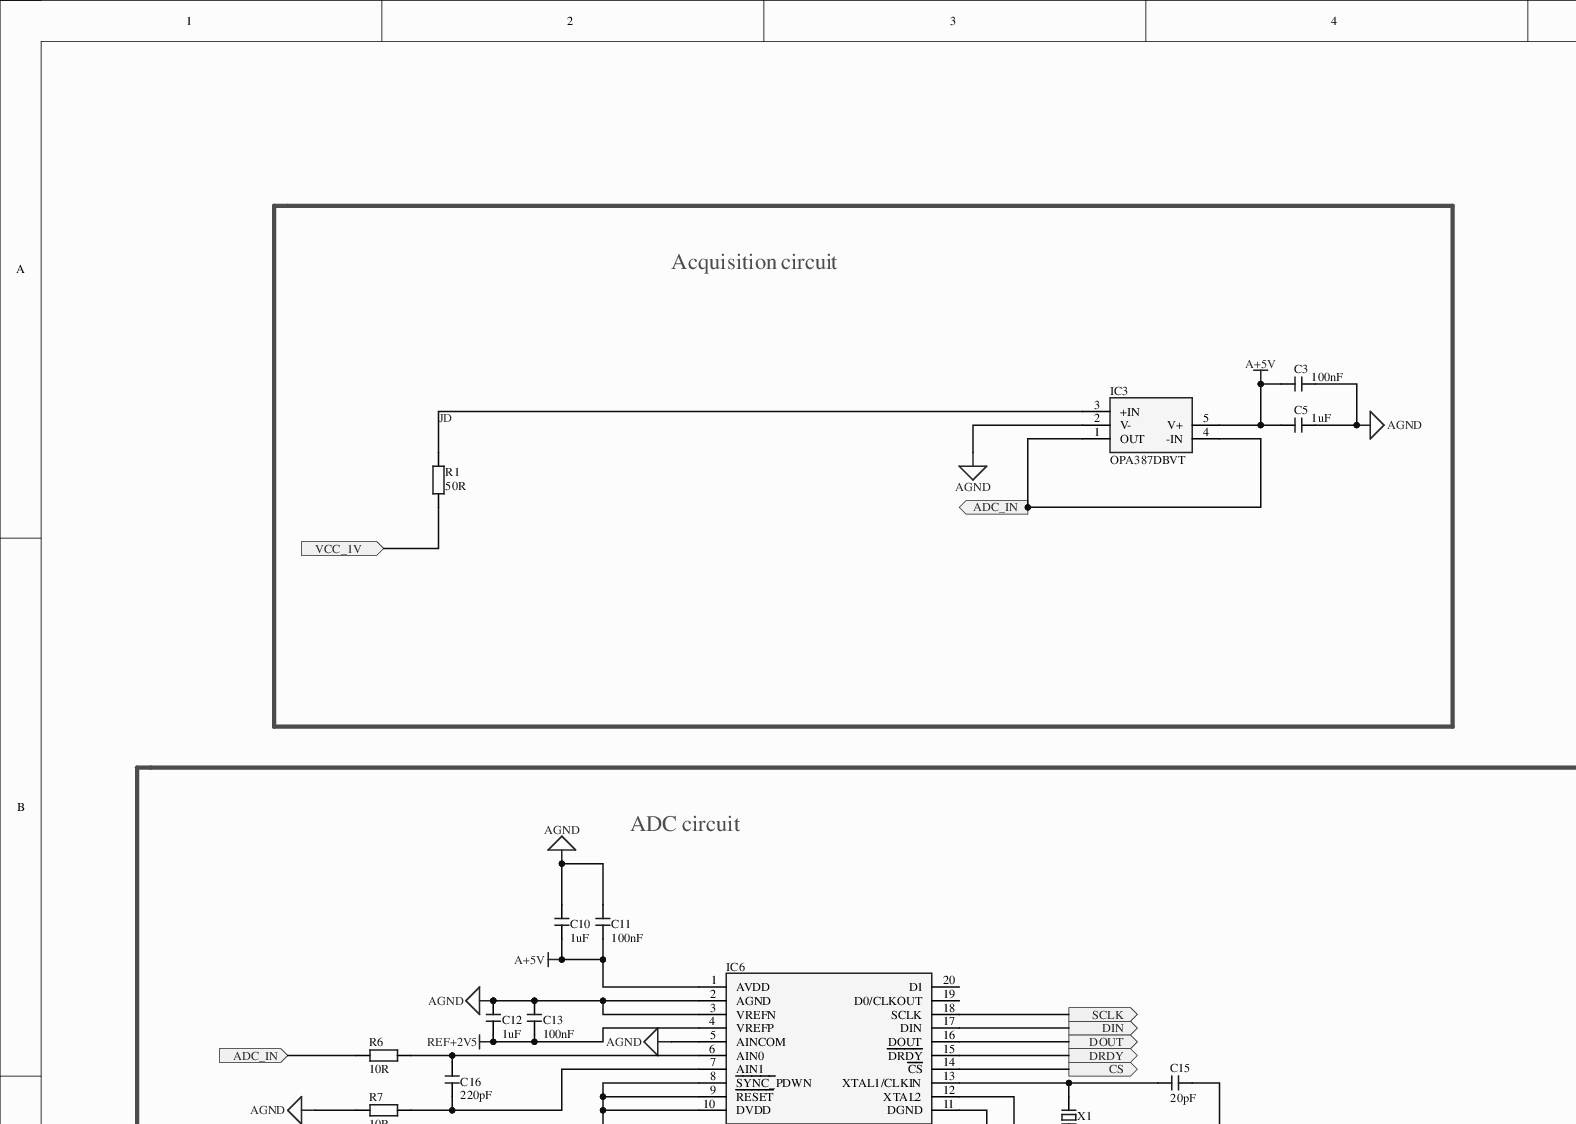
[diagram p0: MISC82306-4.SchDoc, top left]
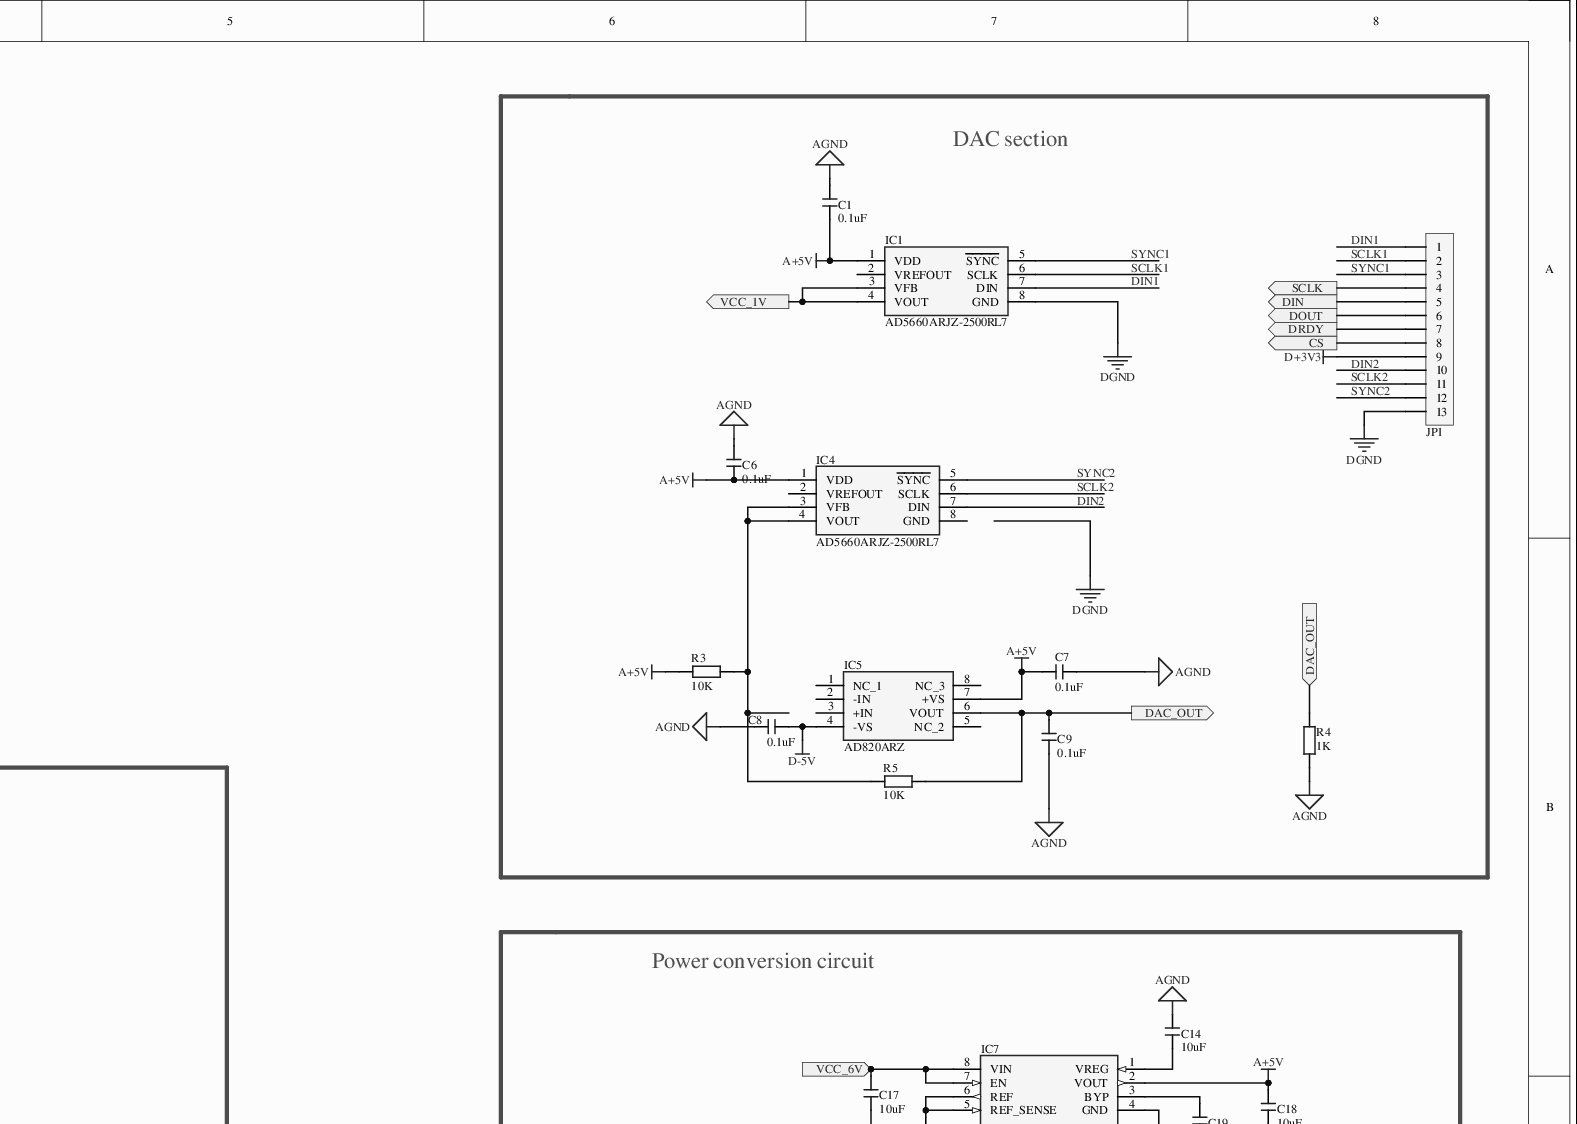
[diagram p1: MISC82306-4.SchDoc, top right]
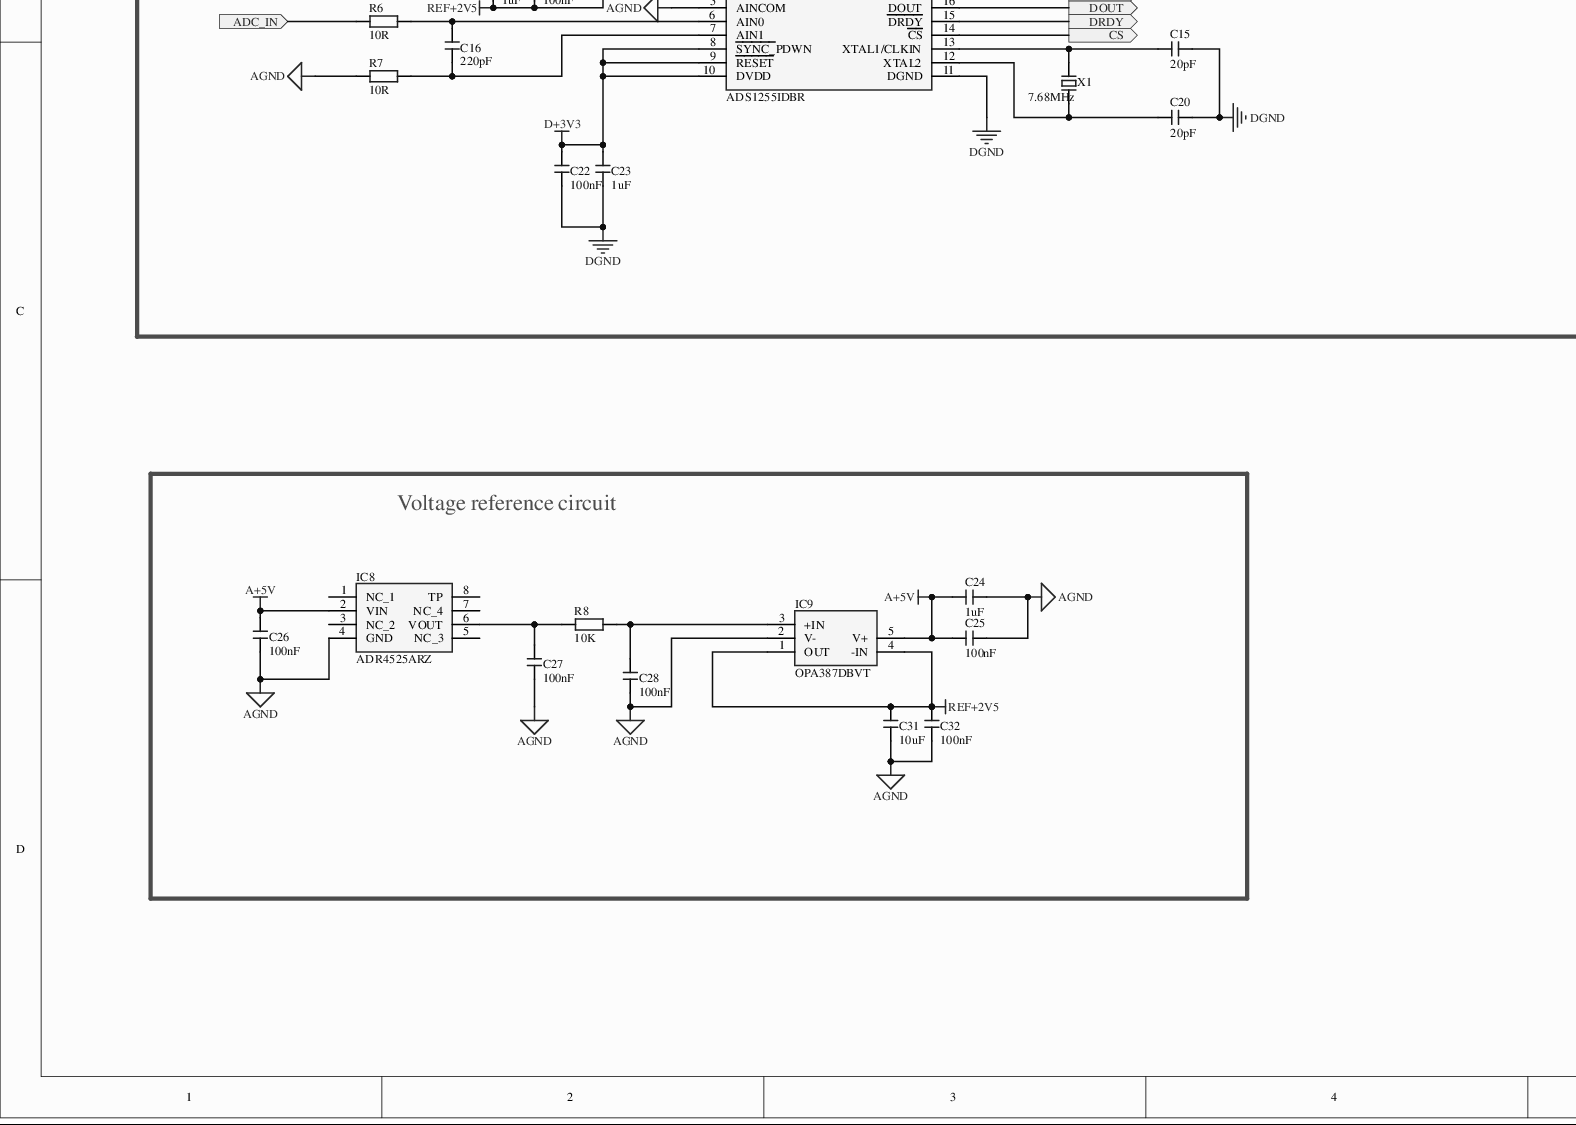
[diagram p2: MISC82306-4.SchDoc, bottom left]
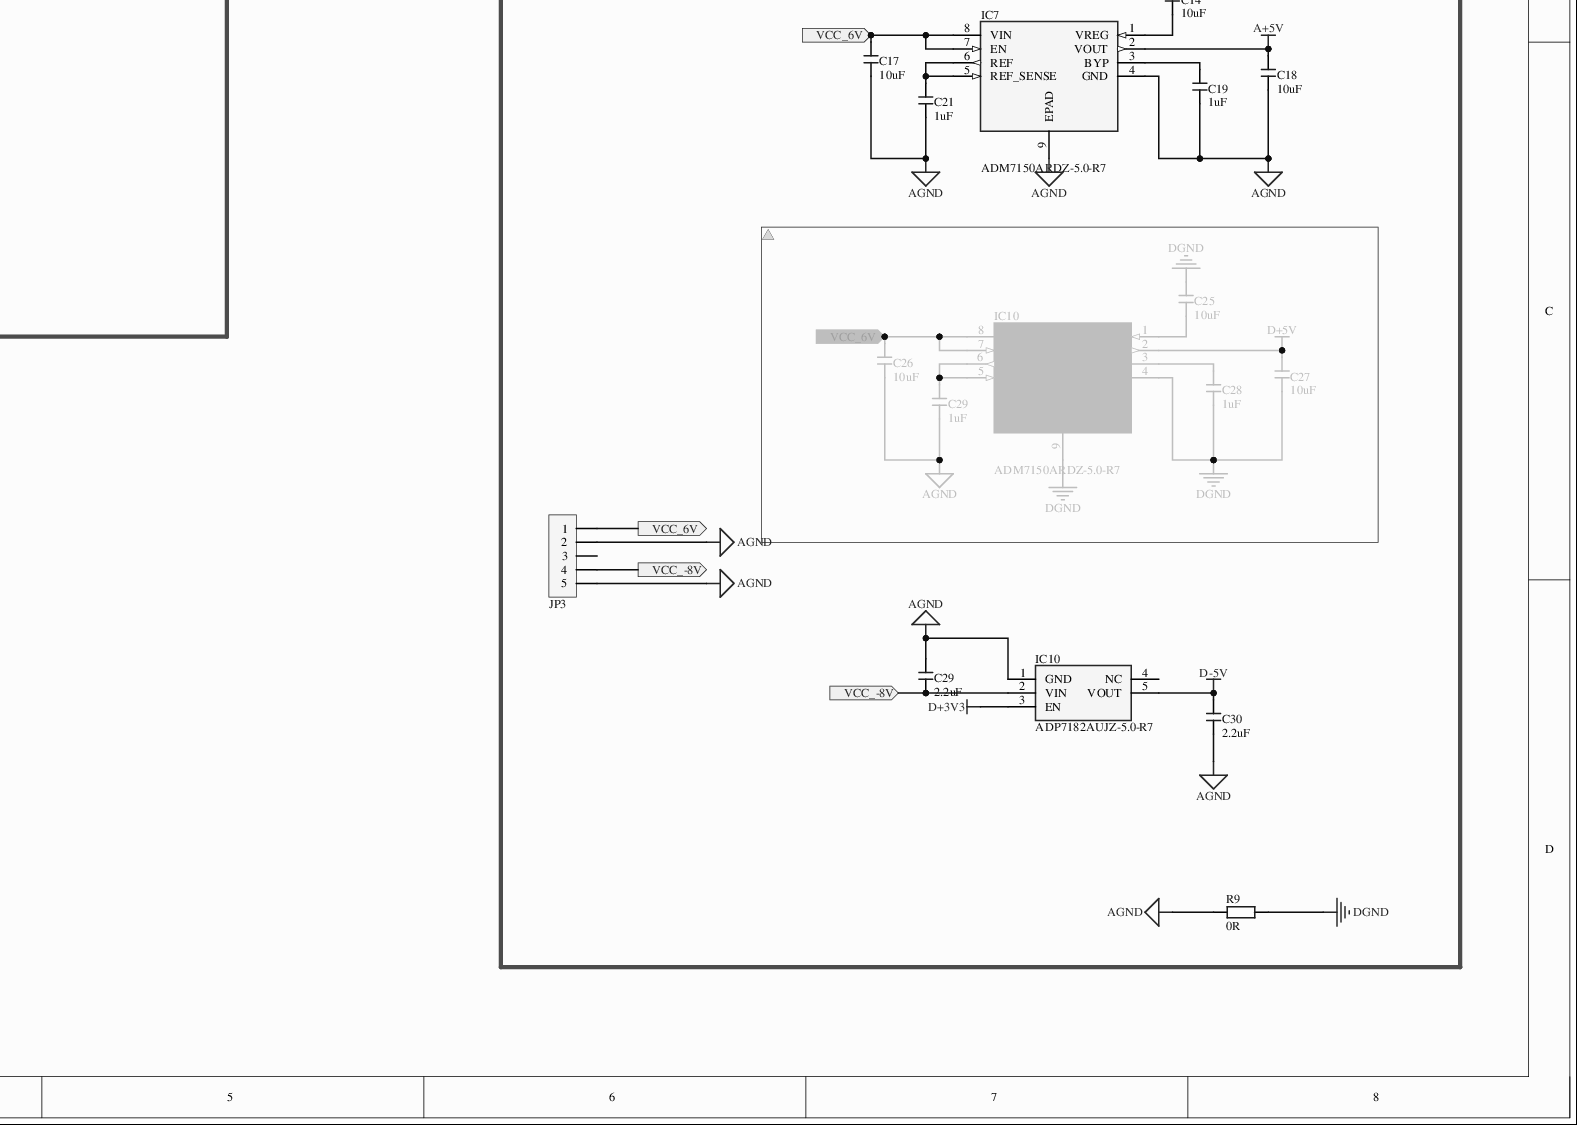
[diagram p3: MISC82306-4.SchDoc, bottom right]
# Altium project MISC82306-7.PrjPcb
1 sheet, 56 parts. Net scope: flat (ports and power ports of the same name join across sheets).
Board file: MISC82306.PcbDoc

## Sheet MISC82306-4.SchDoc
size A2

### Parts
(Parts that share a designator on the sheet are numbered #1, #2 ... from top to bottom, then left to right.)
C1  0.1uF  [C 0603_L]
C3  100nF  [C 0603_L]
C5  1uF  [C 0603_L]
C6  0.1uF  [C 0603_L]
C7  0.1uF  [C 0603_L]
C8  0.1uF  [C 0603_L]
C9  0.1uF  [C 0603_L]
C10  1uF  [C 0603_L]
C11  100nF  [C 0603_L]
C12  1uF  [C 0603_L]
C13  100nF  [C 0603_L]
C14  10uF  [C 0603_L]
C15  20pF  [C 0603_L]
C16  220pF  [C 0805_L]
C17  10uF  [C 0603_L]
C18  10uF  [C 0603_L]
C19  1uF  [C 0603_L]
C20  20pF  [C 0603_L]
C21  1uF  [C 0603_L]
C22  100nF  [C 0603_L]
C23  1uF  [C 0603_L]
C24  1uF  [C 0603_L]
C25#1  10uF  [C 0603_L]  (masked out: inside a compile mask, not in the netlist)
C25#2  100nF  [C 0603_L]
C26#1  10uF  [C 0603_L]  (masked out: inside a compile mask, not in the netlist)
C26#2  100nF  [C 0603_L]
C27#1  10uF  [C 0603_L]  (masked out: inside a compile mask, not in the netlist)
C27#2  100nF  [C 0603_L]
C28#1  1uF  [C 0603_L]  (masked out: inside a compile mask, not in the netlist)
C28#2  100nF  [C 0603_L]
C29#1  1uF  [C 0603_L]  (masked out: inside a compile mask, not in the netlist)
C29#2  2.2uF  [C 0805_L]
C30  2.2uF  [C 0805_L]
C31  10uF  [C 0603_L]
C32  100nF  [C 0603_L]
IC1  AD5660ARJZ-2500RL7  [SOT65P280X145-8N]
IC3  OPA387DBVT  [SOT95P280X100-5N]
IC4  AD5660ARJZ-2500RL7  [SOT65P280X145-8N]
IC5  AD820ARZ  [SOIC127P600X175-8N]
IC6  ADS1255IDBR  [SOP65P780X200-20N]
IC7  ADM7150ARDZ-5.0-R7  [SOIC127P600X175-9N]
IC8  ADR4525ARZ  [SOIC127P600X175-8N]
IC9  OPA387DBVT  [SOT95P280X145-5N]
IC10#1  ADM7150ARDZ-5.0-R7  [SOIC127P600X175-9N]  (masked out: inside a compile mask, not in the netlist)
IC10#2  ADP7182AUJZ-5.0-R7  [SOT95P280X100-5N]
JP1  HDR-1X13  [HDR2.54-LI-13P]  (value not drawn)
JP3  HDR-1X5  [HDR2.54-LI-5P]  (value not drawn)
R1  50R  [R 0805_L]
R3  10K  [R 0603_L]
R4  1K  [R 0603_L]
R5  10K  [R 0603_L]
R6  10R  [R 0603_L]
R7  10R  [R 0603_L]
R8  10K  [R 0805_L]
R9  0R  [R 0805_L]
X1  7.68MHz  [OSC HC-49SMD]

### Blocks framed on the sheet
DAC section: C1 C6-C9 IC1 IC4 IC5 JP1 R3-R5
Acquisition circuit: C3 C5 IC3 R1
ADC circuit: C10-C13 C15 C16 C20 C22 C23 IC6 R6 R7 X1
Power conversion circuit: C14 C17-C19 C21 C25#1 C26#1 C27#1 C28#1 C29#1 C29#2 C30 IC7 IC10#1 IC10#2 JP3 R9
Voltage reference circuit: C24 C25#2 C26#2 C27#2 C28#2 C31 C32 IC8 IC9 R8

### Ports
ADC_IN (in), ADC_IN (out), CS (out), DAC_OUT (in), DAC_OUT (out), DIN (out), DOUT (out), DRDY (out), SCLK (out), VCC_1V (in), VCC_1V (out), VCC_6V (in), VCC_6V (out), VCC_-8V (in), VCC_-8V (out)

### Nets
A+5V: C1.1 C3.1 C5.1 C6.1 C7.1 C10.1 C11.1 C18.1 C24.1 C25#2.1 C26#2.1 IC1.1(VDD) IC3.5(V+) IC4.1(VDD) IC5.7(+VS) IC6.1(AVDD) IC7.2(VOUT) IC8.2(VIN) IC9.5(V+) R3.2
AGND: C1.2 C3.2 C5.2 C6.2 C7.2 C8.1 C9.2 C10.2 C11.2 C12.2 C13.2 C14.2 C17.2 C18.2 C19.2 C21.2 C24.2 C25#2.2 C26#2.2 C27#2.2 C28#2.2 C29#2.1 C30.2 C31.1 C32.1 IC3.2(V-) IC6.2(AGND) IC6.3(VREFN) IC6.5(AINCOM) IC7.4(GND) IC7.9(EPAD) IC8.4(GND) IC9.2(V-) IC10#2.1(GND) JP3.2 JP3.5 R4.1 R7.1 R9.1
D+3V3: C22.1 C23.1 IC6.8(~{SYNC_}PDWN) IC6.9(~{RESET}) IC6.10(DVDD) IC10#2.3(EN) JP1.9
D-5V: C8.2 C30.1 IC5.4(-VS) IC10#2.5(VOUT)
DGND: C15.2 C20.2 C22.2 C23.2 IC1.8(GND) IC6.11(DGND) JP1.13 R9.2
REF+2V5: C12.1 C13.1 C31.2 C32.2 IC6.4(VREFP) IC9.1(OUT) IC9.4(-IN)
DIN1: IC1.7(DIN) JP1.1
DIN2: IC4.7(DIN) JP1.10
JD: IC3.3(+IN) R1.2
SCLK1: IC1.6(SCLK) JP1.2
SCLK2: IC4.6(SCLK) JP1.11
SYNC1: IC1.5(~{SYNC}) JP1.3
SYNC2: IC4.5(~{SYNC}) JP1.12
NetC9_1: C9.1 IC5.6(VOUT) R4.2 R5.1 ; port DAC_OUT
NetC14_1: C14.1 IC7.1(VREG)
NetC15_1: C15.1 IC6.13(XTAL1/CLKIN) X1.2
NetC16_1: C16.1 IC6.7(AIN1) R7.2
NetC16_2: C16.2 IC6.6(AIN0) R6.2
NetC17_1: C17.1 IC7.7(EN) IC7.8(VIN) JP3.1 ; port VCC_6V
NetC19_1: C19.1 IC7.3(BYP)
NetC20_1: C20.1 IC6.12(XTAL2) X1.1
NetC21_1: C21.1 IC7.5(REF_SENSE) IC7.6(REF)
NetC27#2_1: C27#2.1 IC8.6(VOUT) R8.1
NetC28#2_1: C28#2.1 IC9.3(+IN) R8.2
NetC29#2_2: C29#2.2 IC10#2.2(VIN) JP3.4 ; port VCC_-8V
NetIC1_3: IC1.3(VFB) IC1.4(VOUT) R1.1 ; port VCC_1V
NetIC3_1: IC3.1(OUT) IC3.4(-IN) R6.1 ; port ADC_IN
NetIC4_3: IC4.3(VFB) IC4.4(VOUT) R3.1 R5.2
NetIC6_14: IC6.14(~{CS}) JP1.8 ; port CS
NetIC6_15: IC6.15(~{DRDY}) JP1.7 ; port DRDY
NetIC6_16: IC6.16(DOUT) JP1.6 ; port DOUT
NetIC6_17: IC6.17(DIN) JP1.5 ; port DIN
NetIC6_18: IC6.18(SCLK) JP1.4 ; port SCLK

Not connected (* = marked no-connect by the designer): IC1 2(VREFOUT)*; IC4 2(VREFOUT)* 8(GND); IC5 1(NC_1) 2(-IN) 3(+IN) 5(NC_2) 8(NC_3); IC6 19(D0/CLKOUT)* 20(D1)*; IC8 1(NC_1) 3(NC_2) 5(NC_3) 7(NC_4) 8(TP); IC10#2 4(NC); JP3 3

### Library data of the parts
C1 C3 C5-C24 C25#1 C25#2 C26#1 C26#2 C27#1 C27#2 C28#1 C28#2 C29#1 C29#2 C30-C32 = C: Non-polar chip capacitor; 版权归属: COMPANY_A; BOM名称: Non-polar chip capacitor
IC1 = AD5620ARJZ-1500RL7: Integrated Circuit; Manufacturer_Name: Analog Devices; Datasheet Link: http://www.analog.com/media/en/technical-documentation/data-sheets/AD5620_5640_5660.pdf; Height: 1.45mm; Manufacturer_Part_Number: AD5620ARJZ-1500RL7; Mouser Part Number: 584-AD5620ARJZ1500R7; Mouser Price/Stock: https://www.mouser.com/Search/Refine.aspx?Keyword=584-AD5620ARJZ1500R7; Arrow Part Number: AD5620ARJZ-1500RL7; Arrow Price/Stock: https://www.arrow.com/en/products/ad5620arjz-1500rl7/analog-devices
IC3 IC9 = OPA387DBVT: Integrated Circuit; Manufacturer_Name: Texas Instruments; Datasheet Link: https://www.ti.com/lit/ds/symlink/opa387.pdf?HQS=dis-dk-null-digikeymode-dsf-pf-null-wwe&ts=1637562626479; Height: 1.45mm; Manufacturer_Part_Number: OPA387DBVT; Mouser Part Number: 595-OPA387DBVT; Mouser Price/Stock: https://www.mouser.co.uk/ProductDetail/Texas-Instruments/OPA387DBVT?qs=A6eO%252BMLsxmQQsPBKwQXoLw%3D%3D; Arrow Part Number: OPA387DBVT; Arrow Price/Stock: https://www.arrow.com/en/products/opa387dbvt/texas-instruments?region=nac
IC4 = AD5660ARJZ-2500RL7: Integrated Circuit; Manufacturer_Name: Analog Devices; Datasheet Link: https://datasheet.datasheetarchive.com/originals/distributors/Datasheets-4/DSA-70063.pdf; Height: 1.45mm; Manufacturer_Part_Number: AD5660ARJZ-2500RL7; Mouser Part Number: 584-AD5660ARJZ2500R7; Mouser Price/Stock: https://www.mouser.co.uk/ProductDetail/Analog-Devices/AD5660ARJZ-2500RL7?qs=NmRFExCfTkHCkFJjCcAiaw%3D%3D; Arrow Part Number: AD5660ARJZ-2500RL7; Arrow Price/Stock: https://www.arrow.com/en/products/ad5660arjz-2500rl7/analog-devices?region=nac
IC5 = AD820ARZ: Integrated Circuit; Manufacturer_Name: Analog Devices; Datasheet Link: http://www.analog.com/static/imported-files/data_sheets/AD820.pdf; Height: 1.75mm; Manufacturer_Part_Number: AD820ARZ; Mouser Part Number: 584-AD820ARZ; Mouser Price/Stock: https://www.mouser.co.uk/ProductDetail/Analog-Devices/AD820ARZ?qs=%2FtpEQrCGXCz5MA49ylSgWA%3D%3D; Arrow Part Number: AD820ARZ; Arrow Price/Stock: https://www.arrow.com/en/products/ad820arz/analog-devices?region=europe
IC6 = ADS1255IDBR: Integrated Circuit; Manufacturer_Name: Texas Instruments; Datasheet Link: http://www.ti.com/lit/gpn/ads1255; Height: 2mm; Manufacturer_Part_Number: ADS1255IDBR; Mouser Part Number: 595-ADS1255IDBR; Mouser Price/Stock: https://www.mouser.co.uk/ProductDetail/Texas-Instruments/ADS1255IDBR?qs=RaXRGs7zCv5vXRtM5faqvA%3D%3D; Arrow Part Number: ADS1255IDBR; Arrow Price/Stock: https://www.arrow.com/en/products/ads1255idbr/texas-instruments?region=nac
IC7 IC10#1 = ADM7150ARDZ-5.0-R7: Integrated Circuit; Manufacturer_Name: Analog Devices; Datasheet Link: https://componentsearchengine.com/Datasheets/1/ADM7150ARDZ-5.0-R7.pdf; Height: 1.75mm; Manufacturer_Part_Number: ADM7150ARDZ-5.0-R7; Mouser Part Number: 584-ADM7150ARDZ5.0R7; Mouser Price/Stock: https://www.mouser.co.uk/ProductDetail/Analog-Devices/ADM7150ARDZ-5.0-R7?qs=J50fqX%2Fl9iqoesMUO5aNgw%3D%3D; Arrow Part Number: ADM7150ARDZ-5.0-R7; Arrow Price/Stock: https://www.arrow.com/en/products/adm7150ardz-5.0-r7/analog-devices?region=nac
IC8 = ADR4525ARZ: Integrated Circuit; Manufacturer_Name: Analog Devices; Datasheet Link: https://www.analog.com/ADR4525/datasheet; Height: 1.75mm; Manufacturer_Part_Number: ADR4525ARZ; Mouser Part Number: 584-ADR4525ARZ; Mouser Price/Stock: https://www.mouser.co.uk/ProductDetail/Analog-Devices/ADR4525ARZ?qs=WIvQP4zGangC7PeS%252B5s%2F2Q%3D%3D; Arrow Part Number: ADR4525ARZ; Arrow Price/Stock: https://www.arrow.com/en/products/adr4525arz/analog-devices?region=europe
IC10#2 = ADP7182AUJZ-5.0-R7: Integrated Circuit; Manufacturer_Name: Analog Devices; Datasheet Link: https://www.analog.com/media/en/technical-documentation/data-sheets/ADP7182.pdf; Height: 1mm; Manufacturer_Part_Number: ADP7182AUJZ-5.0-R7; Mouser Part Number: 584-ADP7182AUJZ5.0R7; Mouser Price/Stock: https://www.mouser.co.uk/ProductDetail/Analog-Devices/ADP7182AUJZ-5.0-R7?qs=J50fqX%2Fl9ioiLvDNRlnZkg%3D%3D; Arrow Part Number: ADP7182AUJZ-5.0-R7; Arrow Price/Stock: https://www.arrow.com/en/products/adp7182aujz-5.0-r7/analog-devices?region=nac
JP1 = Header 13: 13P connector; 版权归属: COMPANY_A; BOM名称: 13P connector
JP3 = Header 5: 5P connector; 版权归属: COMPANY_A; BOM名称: 5P connector
R1 R3 R5 = R: PTFR0603B100RN9; BOM名称: Chip resistor; 版权归属: COMPANY_A
R4 R6-R9 = R: Chip resistor; 版权归属: COMPANY_A; BOM名称: Chip resistor
X1 = XTAL-2P: 2-pin passive crystal oscillator; 版权归属: COMPANY_A; BOM名称: 2-pin passive crystal oscillator